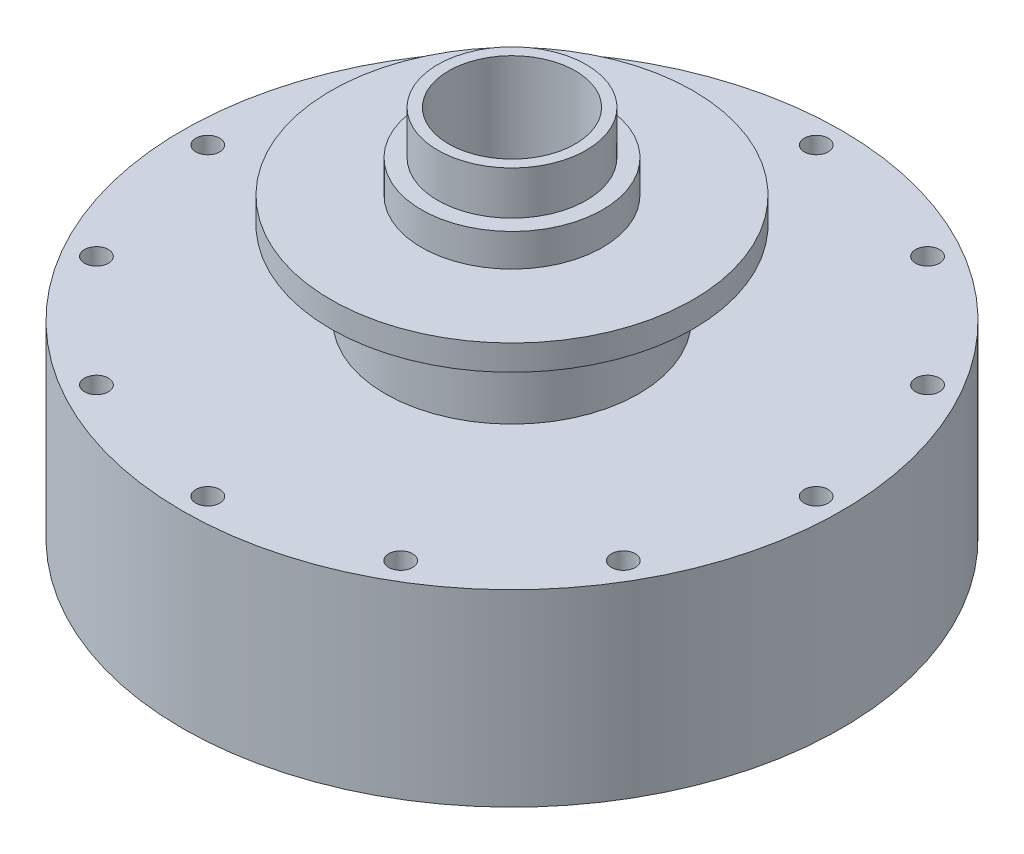
from build123d import *

# Parameters (mm, degrees)
SKETCH_2_R             = 17.5
CUT_EXTRUDE_1_DEPTH    = 169.650526237
HOLE_WIZARD_M6_1_D     = 6.6
HOLE_WIZARD_M8_1_D     = 6.8
HOLE_WIZARD_M8_1_DEPTH = 19.75
HOLE_WIZARD_M8_1_TIP   = 2.042926105
SKETCH_9_W             = 15
SKETCH_9_H             = 23


with BuildPart() as part:
    # 草图1 → 旋转1 (revolve)
    with BuildSketch(Plane.XY, mode=Mode.PRIVATE) as revolve_1_sk:
        Polygon((0, 0), (70, 0), (70, 6), (91, 6), (91, 58), (50, 58), (50, 88), (25, 88), (25, 97), (20.5, 97), (20.5, 109), (0, 109), align=None)
    revolve(revolve_1_sk.sketch.rotate(Axis((0, 0, 0), (0, 1, 0)), 90), axis=Axis((0, 0, 0), (0, 1, 0)))

    # 草图2 → 切除-拉伸1 (cut, through all)
    with BuildSketch(Plane(origin=(0, 109, 0), x_dir=(1, 0, 0), z_dir=(0, 1, 0))):
        with Locations(Location((0, 0, 0), (0, 0, 270))):
            Circle(SKETCH_2_R)
    extrude(amount=-CUT_EXTRUDE_1_DEPTH, mode=Mode.SUBTRACT)

    # M6 间隙孔1 (through all)
    with Locations(Plane(origin=(0, 58, 0), x_dir=(1, 0, 0), z_dir=(0, 1, 0))):
        with Locations((0, 84), (42, 72.746133918), (72.746133918, 42), (84, 0), (72.746133918, -42), (42, -72.746133918), (0, -84), (-42, -72.746133918), (-72.746133918, -42), (-84, 0), (-72.746133918, 42), (-42, 72.746133918)):
            Hole(HOLE_WIZARD_M6_1_D / 2)

    # M8 螺纹孔1
    with Locations(Plane(origin=(0, 0, 0), x_dir=(-1, 0, 0), z_dir=(0, -1, 0))):
        with Locations((0, 58), (41.012193309, 41.012193309), (58, 0), (41.012193309, -41.012193309), (0, -58), (-41.012193309, -41.012193309), (-58, 0), (-41.012193309, 41.012193309)):
            Hole(HOLE_WIZARD_M8_1_D / 2, depth=HOLE_WIZARD_M8_1_DEPTH)
            with Locations((0, 0, -(HOLE_WIZARD_M8_1_DEPTH + HOLE_WIZARD_M8_1_TIP / 2))):  # 118° drill point
                Cone(0, HOLE_WIZARD_M8_1_D / 2, HOLE_WIZARD_M8_1_TIP, mode=Mode.SUBTRACT)

    # 草图9 → 切除-旋转1 (revolve, cut)
    with BuildSketch(Plane.XY, mode=Mode.PRIVATE) as cut_revolve_1_sk:
        with Locations((42.5, 69.5)):
            Rectangle(SKETCH_9_W, SKETCH_9_H)
    revolve(cut_revolve_1_sk.sketch.rotate(Axis((0, 0, 0), (0, -1, 0)), 270), axis=Axis((0, 0, 0), (0, -1, 0)), mode=Mode.SUBTRACT)


solid = part.part
